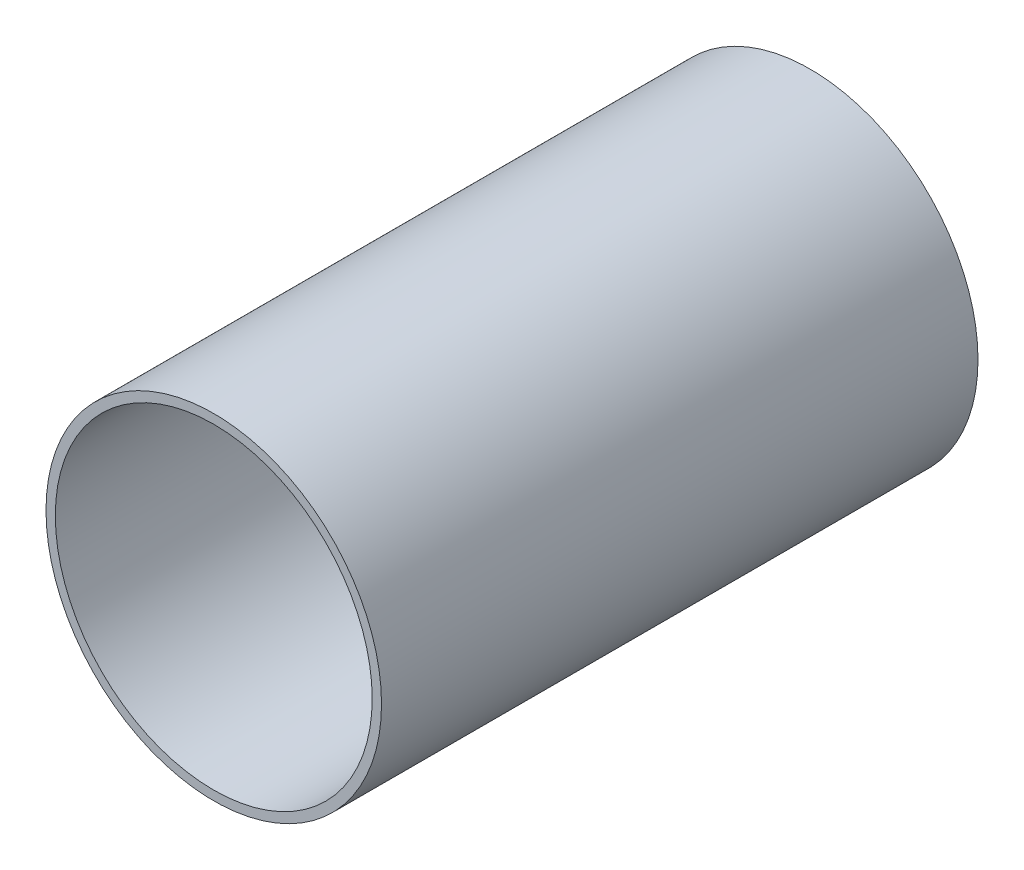
SolidWorks part; units mm, degrees
ref_plane "前视基准面" through (0, 0, 0) normal (0, 0, 1) x (1, 0, 0)
ref_plane "上视基准面" through (0, 0, 0) normal (0, 1, 0) x (1, 0, 0)
ref_plane "右视基准面" through (0, 0, 0) normal (1, 0, 0) x (0, 0, -1)
sketch "草图1" plane through (0, 0, 0) normal (0, 0, 1) x (1, 0, 0)
  circle A0 centre (0, 0) radius 90
  circle A1 centre (0, 0) radius 85
  dimension "D1" = 5
extrude "凸台-拉伸2" add sketch "草图1" along normal blind 320
